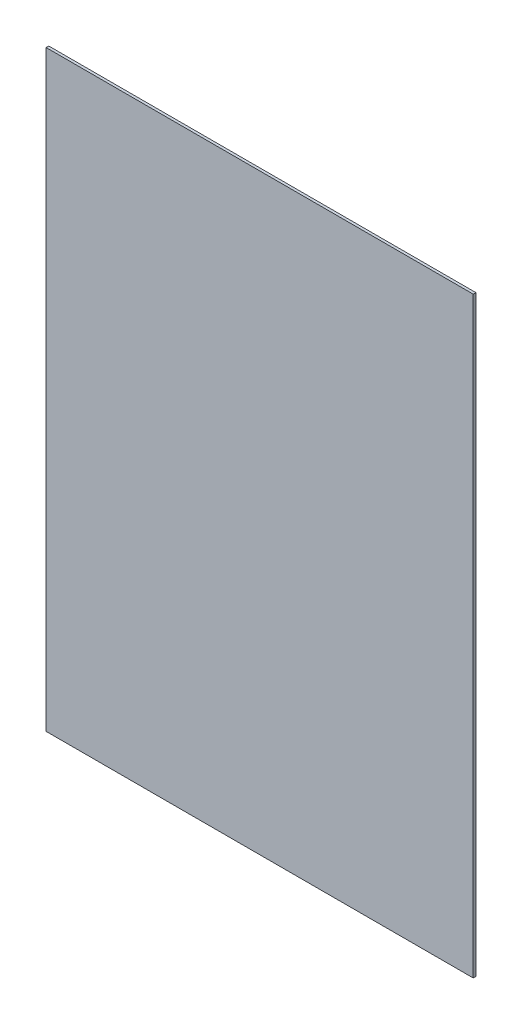
SolidWorks part; units mm, degrees
material "PMMA(有机玻璃)"
ref_plane "前视" through (0, 0, 0) normal (0, 0, 1) x (1, 0, 0)
ref_plane "上视" through (0, 0, 0) normal (0, 1, 0) x (1, 0, 0)
ref_plane "右视" through (0, 0, 0) normal (1, 0, 0) x (0, 0, -1)
sketch "草图1" plane through (0, 0, 0) normal (0, 0, 1) x (1, 0, 0)
  line L1 (-403.5, 559.5) -> (403.5, 559.5)
  line L2 (-403.5, 559.5) -> (-403.5, -559.5)
  line L3 (-403.5, -559.5) -> (403.5, -559.5)
  line L4 (403.5, 559.5) -> (403.5, -559.5)
  line L5 (-403.5, 559.5) -> (403.5, -559.5) construction
  line L6 (-403.5, -559.5) -> (403.5, 559.5) construction
  point P0 (0, 0)
  dimension "D1" = 1119
  dimension "D2" = 807
extrude "凸台-拉伸1" add sketch "草图1" along normal blind 5
